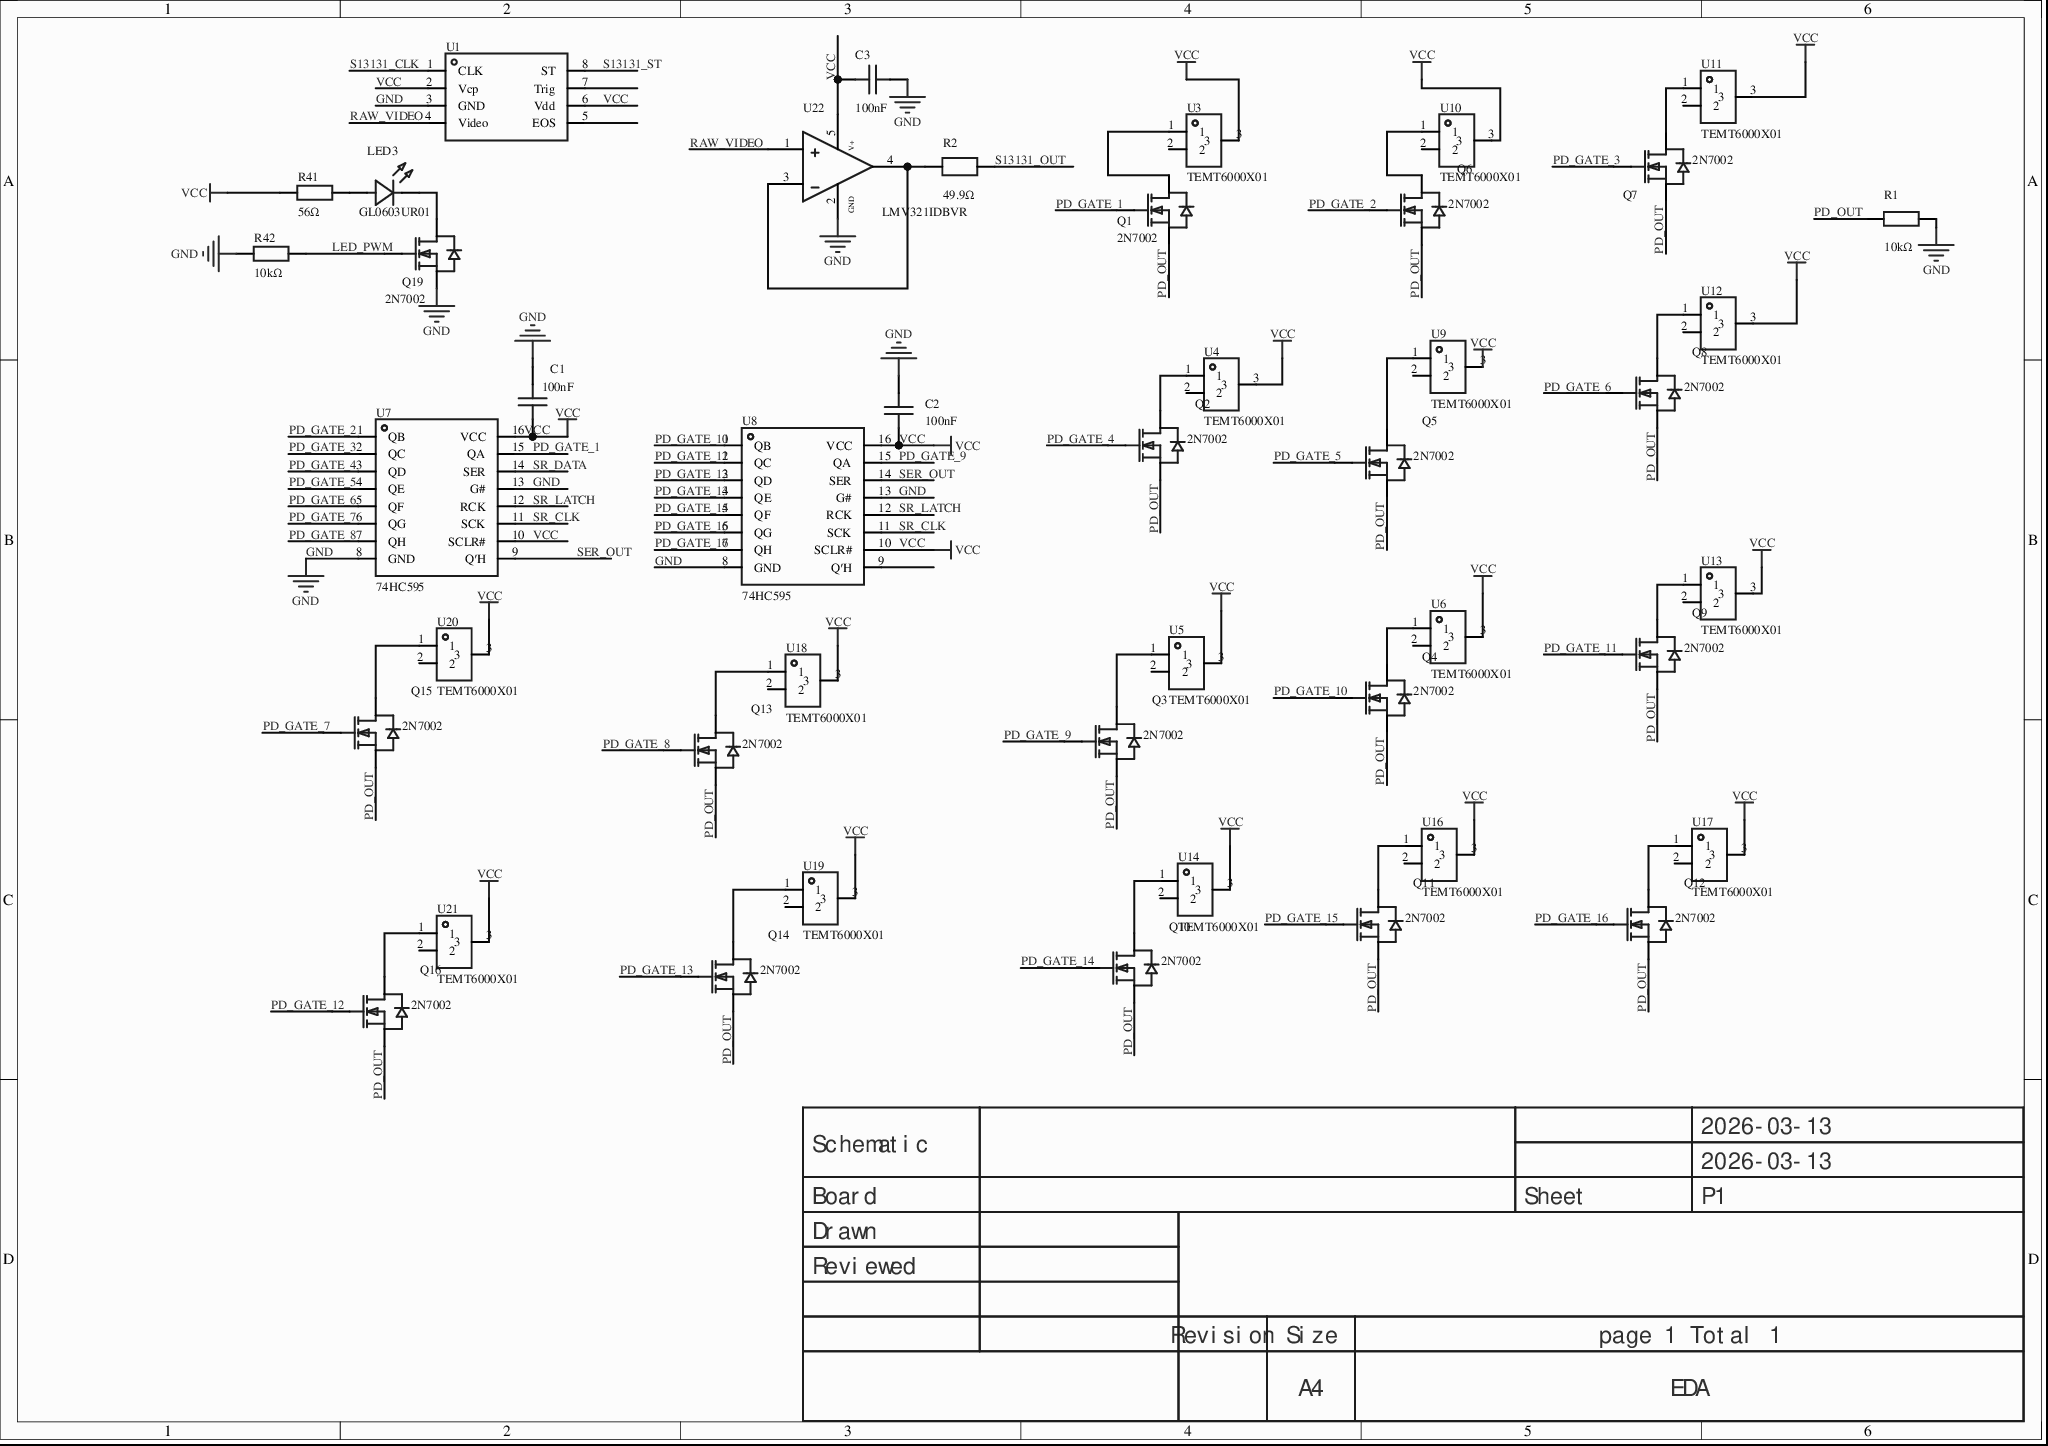
[diagram p0: MISC75432-4.schdoc]
# Altium project MISC75432-2.PrjPcb (part 3 of 3)

## Sheet MISC75432-4.schdoc
size 297 x 209 mm; Version: V1.0; @Project Name: MISC75432; @Update Date: 2026-03-13; @Create Date: 2026-03-13; @Board Name: MISC75432; @Create Time: 12:54:22; @Page Count: 1; @Page No: 1; @Schematic Name: MISC75432; @Update Time: 12:54:22; Size: A4

### Parts
C1  100nF  [C0603]
C2  100nF  [C0603]
C3  100nF  [C0603]
LED3  GL0603UR01  [LED0603-FD]
Q1  2N7002  [SOT-23-3_L2.9-W1.3-P1.90-LS2.4-BR]
Q2  2N7002  [SOT-23-3_L2.9-W1.3-P1.90-LS2.4-BR]
Q3  2N7002  [SOT-23-3_L2.9-W1.3-P1.90-LS2.4-BR]
Q4  2N7002  [SOT-23-3_L2.9-W1.3-P1.90-LS2.4-BR]
Q5  2N7002  [SOT-23-3_L2.9-W1.3-P1.90-LS2.4-BR]
Q6  2N7002  [SOT-23-3_L2.9-W1.3-P1.90-LS2.4-BR]
Q7  2N7002  [SOT-23-3_L2.9-W1.3-P1.90-LS2.4-BR]
Q8  2N7002  [SOT-23-3_L2.9-W1.3-P1.90-LS2.4-BR]
Q9  2N7002  [SOT-23-3_L2.9-W1.3-P1.90-LS2.4-BR]
Q10  2N7002  [SOT-23-3_L2.9-W1.3-P1.90-LS2.4-BR]
Q11  2N7002  [SOT-23-3_L2.9-W1.3-P1.90-LS2.4-BR]
Q12  2N7002  [SOT-23-3_L2.9-W1.3-P1.90-LS2.4-BR]
Q13  2N7002  [SOT-23-3_L2.9-W1.3-P1.90-LS2.4-BR]
Q14  2N7002  [SOT-23-3_L2.9-W1.3-P1.90-LS2.4-BR]
Q15  2N7002  [SOT-23-3_L2.9-W1.3-P1.90-LS2.4-BR]
Q16  2N7002  [SOT-23-3_L2.9-W1.3-P1.90-LS2.4-BR]
Q19  2N7002  [SOT-23-3_L2.9-W1.3-P1.90-LS2.4-BR]
R1  10kΩ  [R0603]
R2  49.9Ω  [R0603]
R41  56Ω  [R0603]
R42  10kΩ  [R0603]
U1  S13131-1536  [BGA-8_L9.1-W2.4_S13131-1536]  (value not drawn)
U3  TEMT6000X01  [SENSORS-SMD_TEMT6000X01]
U4  TEMT6000X01  [SENSORS-SMD_TEMT6000X01]
U5  TEMT6000X01  [SENSORS-SMD_TEMT6000X01]
U6  TEMT6000X01  [SENSORS-SMD_TEMT6000X01]
U7  74HC595  [SOP-16_L9.9-W3.9-P1.27-LS6.0-BL]
U8  74HC595  [SOP-16_L9.9-W3.9-P1.27-LS6.0-BL]
U9  TEMT6000X01  [SENSORS-SMD_TEMT6000X01]
U10  TEMT6000X01  [SENSORS-SMD_TEMT6000X01]
U11  TEMT6000X01  [SENSORS-SMD_TEMT6000X01]
U12  TEMT6000X01  [SENSORS-SMD_TEMT6000X01]
U13  TEMT6000X01  [SENSORS-SMD_TEMT6000X01]
U14  TEMT6000X01  [SENSORS-SMD_TEMT6000X01]
U16  TEMT6000X01  [SENSORS-SMD_TEMT6000X01]
U17  TEMT6000X01  [SENSORS-SMD_TEMT6000X01]
U18  TEMT6000X01  [SENSORS-SMD_TEMT6000X01]
U19  TEMT6000X01  [SENSORS-SMD_TEMT6000X01]
U20  TEMT6000X01  [SENSORS-SMD_TEMT6000X01]
U21  TEMT6000X01  [SENSORS-SMD_TEMT6000X01]
U22  LMV321IDBVR  [SOT-23-5_L3.0-W1.7-P0.95-LS2.8-BR]

### Nets
GND: C1.2 C2.2 C3.2 Q19.2(S) R1.2 R42.2 U1.3(GND) U7.8(GND) U7.13(G#) U8.8(GND) U8.13(G#) U22.2(GND)
VCC: C1.1 C2.1 C3.1 R41.1 U1.2(Vcp) U1.6(Vdd) U3.3 U4.3 U5.3 U6.3 U7.10(SCLR#) U7.16(VCC) U8.10(SCLR#) U8.16(VCC) U9.3 U10.3 U11.3 U12.3 U13.3 U14.3 U16.3 U17.3 U18.3 U19.3 U20.3 U21.3 U22.5(V+)
LED_PWM: Q19.1(G) R42.1
PD_GATE_1: Q1.1(G) U7.15(QA)
PD_GATE_2: Q6.1(G) U7.1(QB)
PD_GATE_3: Q7.1(G) U7.2(QC)
PD_GATE_4: Q2.1(G) U7.3(QD)
PD_GATE_5: Q5.1(G) U7.4(QE)
PD_GATE_6: Q8.1(G) U7.5(QF)
PD_GATE_7: Q15.1(G) U7.6(QG)
PD_GATE_8: Q13.1(G) U7.7(QH)
PD_GATE_9: Q3.1(G) U8.15(QA)
PD_GATE_10: Q4.1(G) U8.1(QB)
PD_GATE_11: Q9.1(G) U8.2(QC)
PD_GATE_12: Q16.1(G) U8.3(QD)
PD_GATE_13: Q14.1(G) U8.4(QE)
PD_GATE_14: Q10.1(G) U8.5(QF)
PD_GATE_15: Q11.1(G) U8.6(QG)
PD_GATE_16: Q12.1(G) U8.7(QH)
PD_OUT: Q1.2(S) Q2.2(S) Q3.2(S) Q4.2(S) Q5.2(S) Q6.2(S) Q7.2(S) Q8.2(S) Q9.2(S) Q10.2(S) Q11.2(S) Q12.2(S) Q13.2(S) Q14.2(S) Q15.2(S) Q16.2(S) R1.1
RAW_VIDEO: U1.4(Video) U22.1(+)
S13131_CLK: U1.1(CLK)
S13131_OUT: R2.2
S13131_ST: U1.8(ST)
SER_OUT: U7.9(Q′H) U8.14(SER)
SR_CLK: U7.11(SCK) U8.11(SCK)
SR_DATA: U7.14(SER)
SR_LATCH: U7.12(RCK) U8.12(RCK)
NetLED3_1: LED3.1(A) R41.2
NetLED3_2: LED3.2(C) Q19.3(D)
NetQ1_3: Q1.3(D) U3.1
NetQ2_3: Q2.3(D) U4.1
NetQ3_3: Q3.3(D) U5.1
NetQ4_3: Q4.3(D) U6.1
NetQ5_3: Q5.3(D) U9.1
NetQ6_3: Q6.3(D) U10.1
NetQ7_3: Q7.3(D) U11.1
NetQ8_3: Q8.3(D) U12.1
NetQ9_3: Q9.3(D) U13.1
NetQ10_3: Q10.3(D) U14.1
NetQ11_3: Q11.3(D) U16.1
NetQ12_3: Q12.3(D) U17.1
NetQ13_3: Q13.3(D) U18.1
NetQ14_3: Q14.3(D) U19.1
NetQ15_3: Q15.3(D) U20.1
NetQ16_3: Q16.3(D) U21.1
NetR2_1: R2.1 U22.3(-) U22.4(OUT)

Not connected (* = marked no-connect by the designer): U1 5(EOS) 7(Trig); U3 2; U4 2; U5 2; U6 2; U8 9(Q′H); U9 2; U10 2; U11 2; U12 2; U13 2; U14 2; U16 2; U17 2; U18 2; U19 2; U20 2; U21 2

### Notes on the sheet
- 2026-03-13
- Schematic
- Board
- Sheet
- P1
- Drawn
- Reviewed
- Revision
- Size
- A4
- page 1 Total 1
- EDA

### Library data of the parts
C1-C3 = CGA0603X7R104K500JT: Capacitance: 100nF; Tolerance: ±10%; Rated voltage: 50V; Temp. coefficient: X7R;; Manufacturer: HRE(芯声); Add into BOM: yes; 3D Model: ac125912035d415993ca9572d50418b1; 3D Model Transform: 62.992,31.496,0,0,0,0,0,0,0; ModelName: C0603_L1.6-W0.8-H0.8; Symbol: CGA0603X7R104K500JT; Device: CGA0603X7R104K500JT; Convert to PCB: yes; Supplier Footprint: 0603; Value: 100nF; LCSC Part Name: 100nF ±10% 50V; Supplier Part: C6119867; Manufacturer Part: CGA0603X7R104K500JT; JLCPCB Part Class: Extended Part; Datasheet: https://example.com/datasheet/CGA0603X7R104K500JT/7062573.html; Supplier: LCSC; Voltage Rating: 50V; Temperature Coefficient: X7R; FootprintName: C0603
LED3 = GL0603UR01: Emitted color: Red; Forward voltage (Vf): 2.4V; Forward current: 20mA; Wavelength: 620nm~625nm; Diode configuration: Discrete diode; Lens color: Clear lens; Luminous intensity: 120mcd; Viewing angle: 120°; Tape mount: Top SMD; Operating temp.: -40℃~+85℃;; Manufacturer: Guiguang light(桂光光电); AddInBom: yes; ModelId: b57d6965da4c4e30afc1a994a1f136ae0819f05c4eef4c71ace90d822a990e87; ModelName: LED0603_Inf; ModelTransform: 60,30,0,0,0,0,0,0,0; Symbol: GL0603UR01; Device: GL0603UR01; LCSC Part Name: 0603 红灯 高亮; SupplierPart: C51933292; ManufacturerPart: GL0603UR01; Supplier Footprint: 0603; JLCPCB Part Class: Extended Part; Datasheet: https://example.com/datasheet/GL0603UR01/54645988.html; Supplier: LCSC; ConvertToPcb: yes; FootprintName: LED0603-FD; Illumination Color: Red; Voltage - Forward(Vf): 2.4V; Forward Current: 20mA; Wavelength - Dominant: 620nm~625nm; Diode Configuration: Discrete diode; Lens Color: Clear lens; Luminous Intensity: 120mcd; Viewing Angle: 120°; Mounting Style: Top SMD; Operating Temperature: -40℃~+85℃
Q1 = 2N7002_C8545: Quantity: 1 N-channel; Drain-source voltage (Vdss): 60V; Continuous drain current (Id): 115mA; On-resistance (RDS(on)): 5Ω@10V; Power dissipation (Pd): 225mW; Threshold voltage (Vgs(th)): 2.5V;; Manufacturer: CJ(江苏长电/长晶); AddInBom: yes; ModelId: c62791f0466c4ae2a892c056b845b0ca0819f05c4eef4c71ace90d822a990e87; ModelName: SOT-23-3P_L2.9-W1.3-H1.0-LS2.4-P0.95; ModelTransform: 98.425,114.173,0,180,0,0,0.0005,-0.0005,0; Input Capacitance(Ciss): 50pF; Reverse Transfer Capacitance (Crss@Vds): 5pF; Symbol: 2N7002; Device: 2N7002_C8545; LCSC Part Name: 1个N沟道 耐压:60V 电流:115mA; SupplierPart: C8545; ManufacturerPart: 2N7002; Supplier Footprint: SOT-23; JLCPCB Part Class: Basic Part; Datasheet: https://example.com/datasheet/2N7002/9040.html; Supplier: LCSC; ConvertToPcb: yes; FootprintName: SOT-23-3_L2.9-W1.3-P1.90-LS2.4-BR; Number: 1 N-channel; Drain to Source Voltage: 60V; Current - Continuous Drain(Id): 115mA; RDS(on): 5Ω@10V; Pd - Power Dissipation: 225mW; Gate Threshold Voltage (Vgs(th)): 2.5V; Operating Temperature: -
Q2-Q16 Q19 = 2N7002_C8545: Quantity: 1 N-channel; Drain-source voltage (Vdss): 60V; Continuous drain current (Id): 115mA; On-resistance (RDS(on)): 5Ω@10V; Power dissipation (Pd): 225mW; Threshold voltage (Vgs(th)): 2.5V;; Manufacturer: CJ(江苏长电/长晶); 3D Model: c62791f0466c4ae2a892c056b845b0ca0819f05c4eef4c71ace90d822a990e87; 3D Model Transform: 98.425,114.173,0,180,0,0,0.0005,-0.0005,0; Input Capacitance(Ciss): 50pF; Reverse Transfer Capacitance (Crss@Vds): 5pF; AddInBom: yes; ModelName: SOT-23-3P_L2.9-W1.3-H1.0-LS2.4-P0.95; Symbol: 2N7002; Device: 2N7002_C8545; LCSC Part Name: 1个N沟道 耐压:60V 电流:115mA; Supplier Part: C8545; Manufacturer Part: 2N7002; Supplier Footprint: SOT-23; JLCPCB Part Class: Basic Part; Datasheet: https://example.com/datasheet/2N7002/9040.html; Supplier: LCSC; Number: 1 N-channel; Drain to Source Voltage: 60V; Current - Continuous Drain(Id): 115mA; RDS(on): 5Ω@10V; Pd - Power Dissipation: 225mW; Gate Threshold Voltage (Vgs(th)): 2.5V; Operating Temperature: -; ConvertToPcb: yes; FootprintName: SOT-23-3_L2.9-W1.3-P1.90-LS2.4-BR
R1 R42 = 0603WAF1002T5E: Resistor type: Thick-film; Resistance: 10kΩ; Tolerance: ±1%; Power: 100mW; Working voltage: 75V; Temp. coefficient: ±100ppm/℃;; Manufacturer: UNI-ROYAL(厚声); Add into BOM: yes; 3D Model: fc143cca1e79419f9cd78b61e9279f08; 3D Model Transform: 31.8897,63.7794,0,90,0,0,0,0,0; Symbol: 0603WAF1002T5E; Device: 0603WAF1002T5E; Convert to PCB: yes; Supplier Footprint: 0603; Value: 10kΩ; LCSC Part Name: 厚膜电阻 10kΩ ±1% 100mW; Supplier Part: C25804; Manufacturer Part: 0603WAF1002T5E; JLCPCB Part Class: Basic Part; Datasheet: https://example.com/datasheet/0603WAF1002T5E/26547.html; Supplier: LCSC; Type: Thick-film resistor; Power(Watts): 100mW; Voltage-Supply(Max): 75V; Temperature Coefficient: ±100ppm/℃; Operating Temperature: -55℃~+155℃; FootprintName: R0603; ModelName: R0603
R2 = FRC0603F49R9TS: Resistor type: Thick-film; Resistance: 49.9Ω; Tolerance: ±1%; Power: 100mW; Working voltage: 75V; Temp. coefficient: ±100ppm/℃;; Manufacturer: FOJAN(富捷); Add into BOM: yes; 3D Model: fc143cca1e79419f9cd78b61e9279f08; 3D Model Transform: 31.8897,63.7794,0,90,0,0,0,0,0; Symbol: FRC0603F49R9TS; Device: FRC0603F49R9TS; Convert to PCB: yes; Supplier Footprint: 0603; Value: 49.9Ω; LCSC Part Name: 49.9Ω ±1% 100mW 厚膜电阻; Supplier Part: C2930110; Manufacturer Part: FRC0603F49R9TS; JLCPCB Part Class: Extended Part; Supplier: LCSC; Type: Thick-film resistor; Power(Watts): 100mW; Voltage-Supply(Max): 75V; Temperature Coefficient: ±100ppm/℃; Operating Temperature: -55℃~+155℃; FootprintName: R0603; ModelName: R0603
R41 = 0603WAF560JT5E: Resistor type: Thick-film; Resistance: 56Ω; Tolerance: ±1%; Power: 100mW; Max working voltage: 75V; Temp. coefficient: ±200ppm/℃;; Manufacturer: UNI-ROYAL(厚声); Add into BOM: yes; 3D Model: fc143cca1e79419f9cd78b61e9279f08; 3D Model Transform: 31.8897,63.7794,0,90,0,0,0,0,0; Symbol: 0603WAF560JT5E; Device: 0603WAF560JT5E; Convert to PCB: yes; Supplier Footprint: 0603; Value: 56Ω; LCSC Part Name: 56Ω ±1% 100mW 厚膜电阻; Supplier Part: C25196; Manufacturer Part: 0603WAF560JT5E; JLCPCB Part Class: Extended Part; Datasheet: https://example.com/upload/public/pdf/source/20200306/C422600_1E6D84923E4A46A82E41ADD87F860B5C.pdf; Supplier: LCSC; Type: Thick-film resistor; Power(Watts): 100mW; Overload Voltage (Max): 75V; Temperature Coefficient: ±200ppm/℃; Operating Temperature Range: -55℃~+155℃; FootprintName: R0603; ModelName: R0603
U1 = S13131-1536: AddInBom: yes; ModelId: ce669231a6704143893a05abd84262fa0819f05c4eef4c71ace90d822a990e87; ModelTransform: 358.267,94.488,0,0,0,0,0,0,0; Symbol: S13131-1536; Device: S13131-1536; LCSC Part Name: S13131-1536; SupplierPart: C5143846; ManufacturerPart: S13131-1536; Supplier Footprint: SMD-8P; JLCPCB Part Class: Extended Part; Supplier: LCSC; ConvertToPcb: yes; FootprintName: BGA-8_L9.1-W2.4_S13131-1536; ModelName: BGA-8_L9.1-W2.4_S13131-1536
U3 = TEMT6000X01: Manufacturer: VISHAY(威世); AddInBom: yes; ModelId: 27ac3504c6184a09b0133c3e249ce6820819f05c4eef4c71ace90d822a990e87; ModelTransform: 157.48,78.74,0,0,0,0,0,0,0; Symbol: TEMT6000X01; Device: TEMT6000X01; LCSC Part Name: TEMT6000X01; SupplierPart: C94098; ManufacturerPart: TEMT6000X01; Supplier Footprint: 1206; JLCPCB Part Class: Extended Part; Datasheet: https://example.com/datasheet/TEMT6000X01/95296.html; Supplier: LCSC; ConvertToPcb: yes; FootprintName: SENSORS-SMD_TEMT6000X01; ModelName: SENSORS-SMD_TEMT6000X01
U4-U6 U9-U14 U16-U21 = TEMT6000X01: Manufacturer: VISHAY(威世); 3D Model: 27ac3504c6184a09b0133c3e249ce6820819f05c4eef4c71ace90d822a990e87; 3D Model Transform: 157.48,78.74,0,0,0,0,0,0,0; AddInBom: yes; Symbol: TEMT6000X01; Device: TEMT6000X01; LCSC Part Name: TEMT6000X01; Supplier Part: C94098; Manufacturer Part: TEMT6000X01; Supplier Footprint: 1206; JLCPCB Part Class: Extended Part; Datasheet: https://example.com/datasheet/TEMT6000X01/95296.html; Supplier: LCSC; ConvertToPcb: yes; FootprintName: SENSORS-SMD_TEMT6000X01; ModelName: SENSORS-SMD_TEMT6000X01
U7 U8 = 74HC595: Function: Serial to serial or parallel; Working voltage: 2V~6V; Clock frequency (fc): 10MHz; Elements: 1; Bits per element: 8;; Manufacturer: GR(国睿); AddInBom: yes; ModelId: ed96d47c1e844792b3e705d722a1a1fa0819f05c4eef4c71ace90d822a990e87; ModelTransform: 389.763,236.22,0,0,0,0,0,0,0; Number of Elements: 1; Number of Bits per Element: 8; Output Type: Tri-state; Propagation Delay: 100ns@5V,50pF; Symbol: 74HC595; Device: 74HC595; LCSC Part Name: 8位CMOS移位寄存器; SupplierPart: C18164493; ManufacturerPart: 74HC595; Supplier Footprint: SOP-16; JLCPCB Part Class: Extended Part; Datasheet: https://example.com/datasheet/74HC595/19305556.html; Supplier: LCSC; ConvertToPcb: yes; FootprintName: SOP-16_L9.9-W3.9-P1.27-LS6.0-BL; ModelName: SOP-16_L9.9-W3.9-P1.27-LS6.0-BL; Voltage - Supply: 2V~6V; Clock Frequency: 10MHz; Series: 74HC; Operating Temperature: -40℃~+85℃
U22 = LMV321IDBVR_C7972: Amplifiers: Single; Rail-to-rail: Rail-to-rail output; Gain-bandwidth product (GBP): 1MHz; Input offset voltage (Vos): 7mV; Slew rate (SR): 1V/us; Input bias current (Ib): 11nA;; Manufacturer: TI(德州仪器); AddInBom: yes; ModelId: 0a2a1b8f50944f73965918ad6e5fe1670819f05c4eef4c71ace90d822a990e87; ModelName: SOT-23-5_L2.9-W1.6-H1.1-LS2.8-P0.95; ModelTransform: 114.173,109.636,0,180,0,0,0,0,0; Maximum Power Supply Range (Vdd-Vss): 5.5V; Input Offset Voltage Drift(Vos TC): 9uV/℃; Input Offset Current(Ios): 5nA; Noise density(eN): 46nV/√Hz@1kHz; Common Mode Rejection Ratio(CMRR): 63dB; Quiescent Current: 170uA; Output Current: 5mA; Single supply: 2.7V~5.5V; Symbol: LMV321IDBVR; Device: LMV321IDBVR_C7972; LCSC Part Name: 低电压轨到轨输出运算放大器; SupplierPart: C7972; ManufacturerPart: LMV321IDBVR; Supplier Footprint: SOT-23-5; JLCPCB Part Class: Extended Part; Supplier: LCSC; ConvertToPcb: yes; FootprintName: SOT-23-5_L3.0-W1.7-P0.95-LS2.8-BR; Number of Channels: Single; Rail to Rail: Rail-to-rail output; Gain Bandwidth Product: 1MHz; Vos - Input Offset Voltage: 7mV; Slew Rate: 1V/us; Ib - Input Bias Current: 11nA; Input offset current drift(Ios TC): -; Operating Temperature: -40℃~+125℃

## Nets that join several sheets
GND: MISC75432-3 (83 pins), MISC75432-4 (12 pins)
VCC: MISC75432-3 (19 pins), MISC75432-4 (27 pins)
LED_PWM: MISC75432-3 (U15.12), MISC75432-4 (Q19.1 R42.1)
PD_OUT: MISC75432-3 (U15.7), MISC75432-4 (17 pins)
S13131_CLK: MISC75432-3 (R12.1), MISC75432-4 (U1.1)
S13131_OUT: MISC75432-3 (U15.6), MISC75432-4 (R2.2)
S13131_ST: MISC75432-3 (R11.1), MISC75432-4 (U1.8)
SR_CLK: MISC75432-3 (R10.1), MISC75432-4 (U7.11 U8.11)
SR_DATA: MISC75432-3 (R8.2), MISC75432-4 (U7.14)
SR_LATCH: MISC75432-3 (R9.2), MISC75432-4 (U7.12 U8.12)